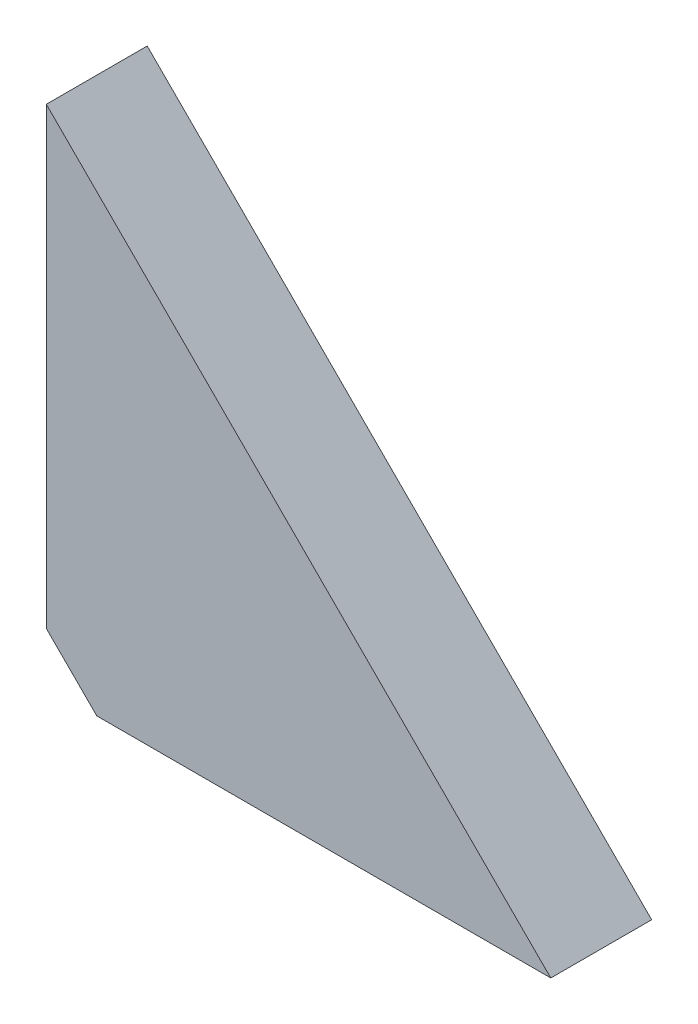
from build123d import *

# Parameters (mm, degrees)
BOSS_EXTRUDE1_DEPTH = 5
CHAMFER1_SIZE       = 5


with BuildPart() as part:
    # Sketch1 → Boss-Extrude1 (new, symmetric)
    with BuildSketch(Plane.XY):
        Polygon((0, 0), (0, 50), (50, 0), align=None)
    extrude(amount=BOSS_EXTRUDE1_DEPTH, both=True)

    # Chamfer1
    chamfer1_edges = [part.edges().sort_by_distance(p)[0] for p in [
        (0, 0, 0),
    ]]
    chamfer(chamfer1_edges, length=CHAMFER1_SIZE)


solid = part.part
